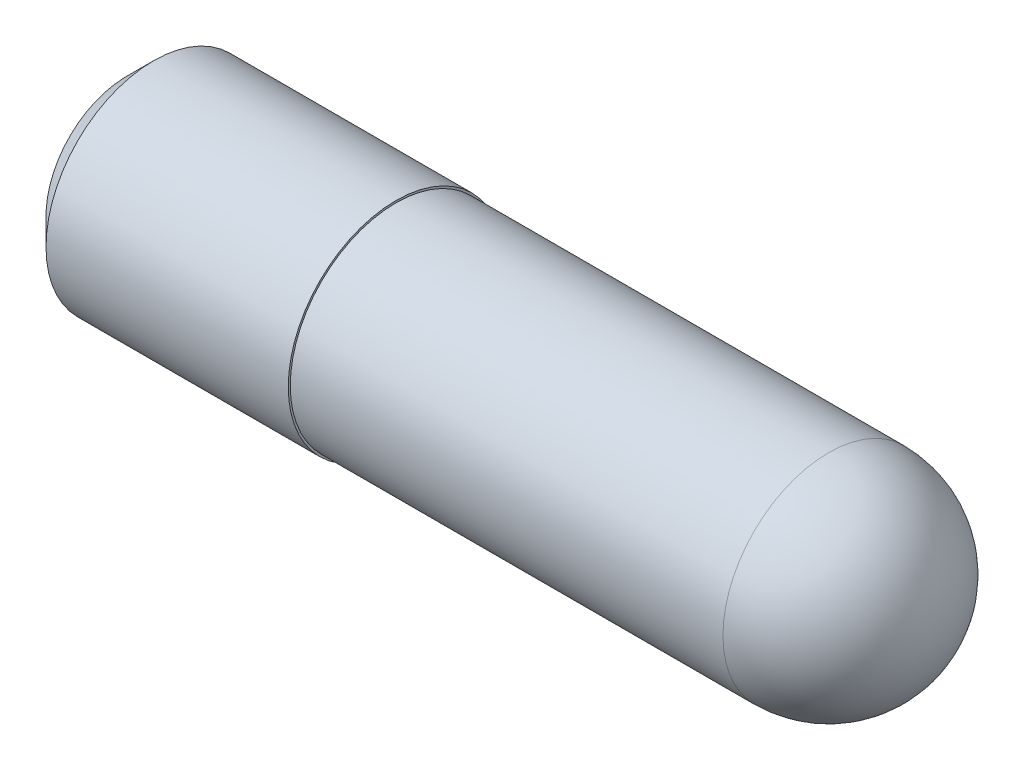
SolidWorks part; units mm, degrees
material "SUS304"
ref_plane "前视基准面" through (0, 0, 0) normal (0, 0, 1) x (1, 0, 0)
ref_plane "上视基准面" through (0, 0, 0) normal (0, 1, 0) x (1, 0, 0)
ref_plane "右视基准面" through (0, 0, 0) normal (1, 0, 0) x (0, 0, -1)
sketch "草图1" plane through (0, 0, 0) normal (1, 0, 0) x (0, 0, -1)
  circle A0 centre (0, 0) radius 4
  dimension "D1" = 8
extrude "凸台-拉伸1" add sketch "草图1" along normal blind 10
sketch "草图2" plane through (10, 0, 0) normal (1, 0, 0) x (0, 0, -1)
  circle A0 centre (0, 0) radius 3.925
  dimension "D1" = 7.85
extrude "凸台-拉伸2" add sketch "草图2" along normal blind 20
fillet "圆角1" radius 3.925 1 edges at (30, 0, -3.925)
chamfer "倒角1" distance 1 angle 45 1 edges at (0, 0, -4)
